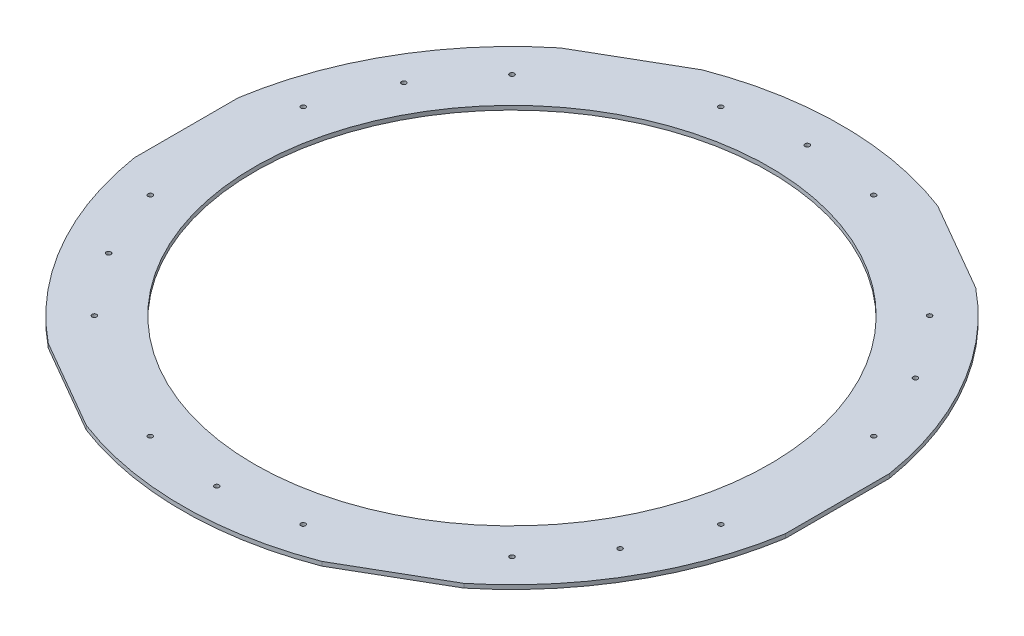
SolidWorks part; units mm, degrees
material "Q235B"
ref_plane "Front Plane" through (0, 0, 0) normal (0, 0, 1) x (1, 0, 0)
ref_plane "Top Plane" through (0, 0, 0) normal (0, 1, 0) x (1, 0, 0)
ref_plane "Right Plane" through (0, 0, 0) normal (1, 0, 0) x (0, 0, -1)
sketch "Sketch1" plane through (0, 0, 0) normal (0, 1, 0) x (1, 0, 0)
  circle A0 centre (0, 0) radius 480
  circle A1 centre (0, 0) radius 375
  dimension "D1" = 960
  dimension "D2" = 750
extrude "Boss-Extrude1" add sketch "Sketch1" along normal blind 6
sketch "Sketch2" plane through (0, 0, 0) normal (0, 1, 0) x (1, 0, 0)
  line L0 (0, 0) -> (0, -480) construction
  line L1 (-474, -250) -> (-486, -250)
  line L2 (-474, -250) -> (-474, 250)
  line L3 (-474, 250) -> (-486, 250)
  line L4 (-486, -250) -> (-486, 250)
  line L5 (-474, -250) -> (-486, 250) construction
  line L6 (-474, 250) -> (-486, -250) construction
  line L7 (474, 250) -> (486, -250) construction
  line L8 (474, -250) -> (486, 250) construction
  line L9 (486, -250) -> (486, 250)
  line L10 (474, 250) -> (486, 250)
  line L11 (474, -250) -> (474, 250)
  line L12 (474, -250) -> (486, -250)
  circle A0 centre (0, 0) radius 480 construction
  point P0 (-480, 0)
  point P15 (480, 0)
  dimension "D1" = 948
  dimension "D2" = 500
extrude "Cut-Extrude3" cut sketch "Sketch2" along normal up to next
pattern_circular "CirPattern1" count 3 over 360 about axis through (0, 0, 0) along (0, 1, 0) of "Cut-Extrude3"
hole_wizard "M8 Tapped Hole1" positions "Sketch3" profile "Sketch4" tap size "M8" standard "GB" end condition up to next
sketch "Sketch3" plane through (0, 6, 0) normal (0, 1, 0) x (1, 0, 0)
  line L1 (0, 0) -> (111.2922, 415.3481) construction
  line L3 (0, 0) -> (0, 430) construction
  circle A0 centre (0, 0) radius 430
  point P0 (0, 430)
  point P2 (111.2922, 415.3481)
  point P21 (-111.2922, 415.3481)
  point P26 (372.3909, 215)
  point P27 (415.3481, 111.2922)
  point P28 (304.0559, 304.0559)
  point P29 (372.3909, -215)
  point P30 (304.0559, -304.0559)
  point P31 (415.3481, -111.2922)
  point P32 (0, -430)
  point P33 (-111.2922, -415.3481)
  point P34 (111.2922, -415.3481)
  point P35 (-372.3909, -215)
  point P36 (-415.3481, -111.2922)
  point P37 (-304.0559, -304.0559)
  point P38 (-372.3909, 215)
  point P39 (-304.0559, 304.0559)
  point P40 (-415.3481, 111.2922)
  point P41 (0, 0)
  dimension "D1" = 15
  dimension "D2" = 860
  dimension "D3" = 6
sketch "Sketch4" plane through (0, 6, -430) normal (1, 0, 0) x (0, 0, 1)
  line L0 (0, 0) -> (0, 6)
  line L1 (0, 6) -> (3.4, 6)
  line L2 (3.4, 6) -> (3.4, 0)
  line L5 (3.4, 0) -> (0, 0)
  line L11 (0, -6.35) -> (0, 107.95) construction
  dimension "通孔螺纹孔钻头直径" = 6.8
  dimension "通孔螺纹孔钻头深度" = 6
cosmetic thread "CosmeticThread1" parameters "D2"=8
cosmetic thread "CosmeticThread2" parameters "D2"=8
cosmetic thread "CosmeticThread3" parameters "D2"=8
cosmetic thread "CosmeticThread4" parameters "D2"=8
cosmetic thread "CosmeticThread5" parameters "D2"=8
cosmetic thread "CosmeticThread6" parameters "D2"=8
cosmetic thread "CosmeticThread7" parameters "D2"=8
cosmetic thread "CosmeticThread8" parameters "D2"=8
cosmetic thread "CosmeticThread9" parameters "D2"=8
cosmetic thread "CosmeticThread10" parameters "D2"=8
cosmetic thread "CosmeticThread11" parameters "D2"=8
cosmetic thread "CosmeticThread12" parameters "D2"=8
cosmetic thread "CosmeticThread13" parameters "D2"=8
cosmetic thread "CosmeticThread14" parameters "D2"=8
cosmetic thread "CosmeticThread15" parameters "D2"=8
cosmetic thread "CosmeticThread16" parameters "D2"=8
cosmetic thread "CosmeticThread17" parameters "D2"=8
cosmetic thread "CosmeticThread18" parameters "D2"=8
